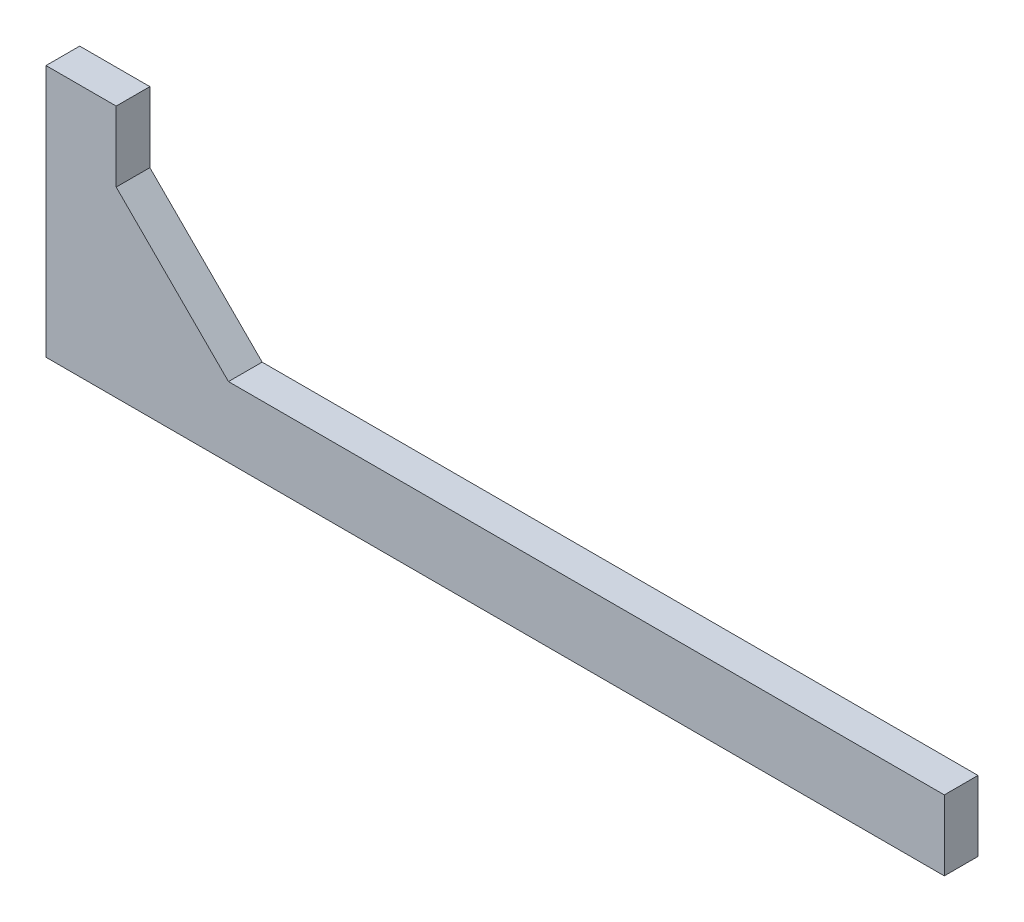
from build123d import *

# Parameters (mm, degrees)
EXTRUDE_1_DEPTH        = 6
HOLE_WIZARD_M8_1_D     = 6.8
HOLE_WIZARD_M8_1_DEPTH = 18.75
HOLE_WIZARD_M8_1_TIP   = 2.042926105
HOLE_WIZARD_M6_1_D     = 5
HOLE_WIZARD_M6_1_DEPTH = 15
HOLE_WIZARD_M6_1_TIP   = 1.502151548


with BuildPart() as part:
    # 草图1 → 凸台-拉伸1 (new, symmetric)
    with BuildSketch(Plane.XY):
        Polygon((0, 0), (0, 90), (25, 90), (25, 65), (65, 25), (320, 25), (320, 0), align=None)
    extrude(amount=EXTRUDE_1_DEPTH, both=True)

    # M8 螺纹孔1
    with Locations(Plane(origin=(0, 75, 0), x_dir=(0, 0, -1), z_dir=(-1, 0, 0))):
        with Locations((0, 0), (0, 50)):
            Hole(HOLE_WIZARD_M8_1_D / 2, depth=HOLE_WIZARD_M8_1_DEPTH)
            with Locations((0, 0, -(HOLE_WIZARD_M8_1_DEPTH + HOLE_WIZARD_M8_1_TIP / 2))):  # 118° drill point
                Cone(0, HOLE_WIZARD_M8_1_D / 2, HOLE_WIZARD_M8_1_TIP, mode=Mode.SUBTRACT)

    # M6 螺纹孔1
    with Locations(Plane(origin=(45, 0, 0), x_dir=(0, 0, -1), z_dir=(0, -1, 0))):
        with Locations((0, 0), (0, 120), (0, 240)):
            Hole(HOLE_WIZARD_M6_1_D / 2, depth=HOLE_WIZARD_M6_1_DEPTH)
            with Locations((0, 0, -(HOLE_WIZARD_M6_1_DEPTH + HOLE_WIZARD_M6_1_TIP / 2))):  # 118° drill point
                Cone(0, HOLE_WIZARD_M6_1_D / 2, HOLE_WIZARD_M6_1_TIP, mode=Mode.SUBTRACT)


solid = part.part
